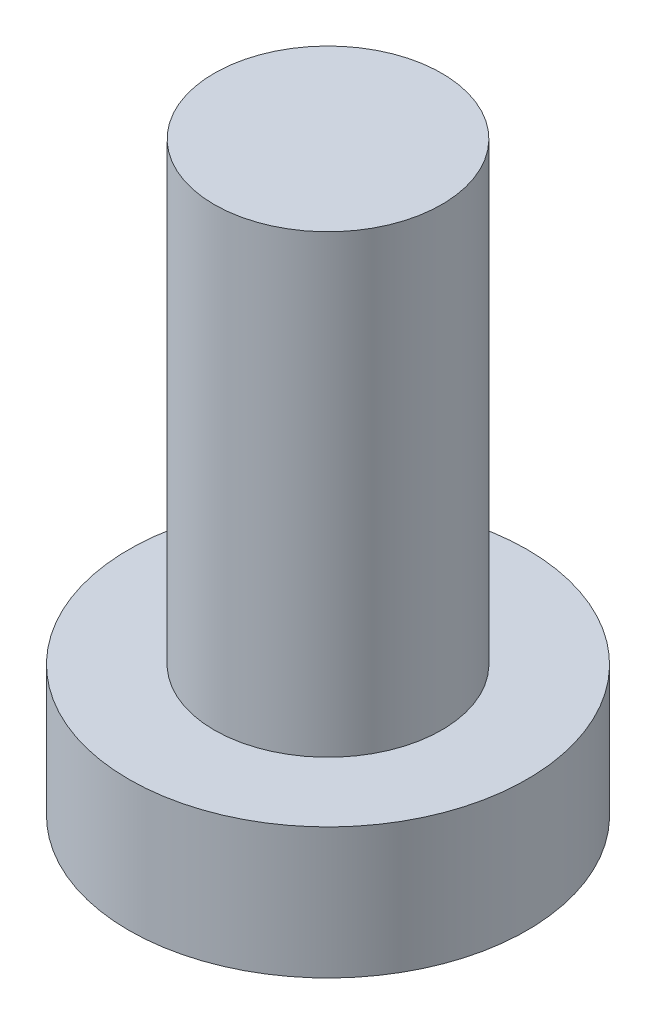
from build123d import *

# Parameters (mm, degrees)
SKETCH_1_R      = 2
EXTRUDE_1_DEPTH = 8
SKETCH_2_R      = 3.5
EXTRUDE_2_DEPTH = 2.3


with BuildPart() as part:
    # 草图1 → 凸台-拉伸1 (new body)
    with BuildSketch(Plane(origin=(0, 0, 0), x_dir=(1, 0, 0), z_dir=(0, 1, 0))):
        with Locations(Location((0, 0, 0), (0, 0, 270))):
            Circle(SKETCH_1_R)
    extrude(amount=EXTRUDE_1_DEPTH)

    # 草图2 → 凸台-拉伸2 (add)
    with BuildSketch(Plane.XZ):
        with Locations(Location((0, 0, 0), (0, 0, 270))):
            Circle(SKETCH_2_R)
    extrude(amount=EXTRUDE_2_DEPTH)


solid = part.part
